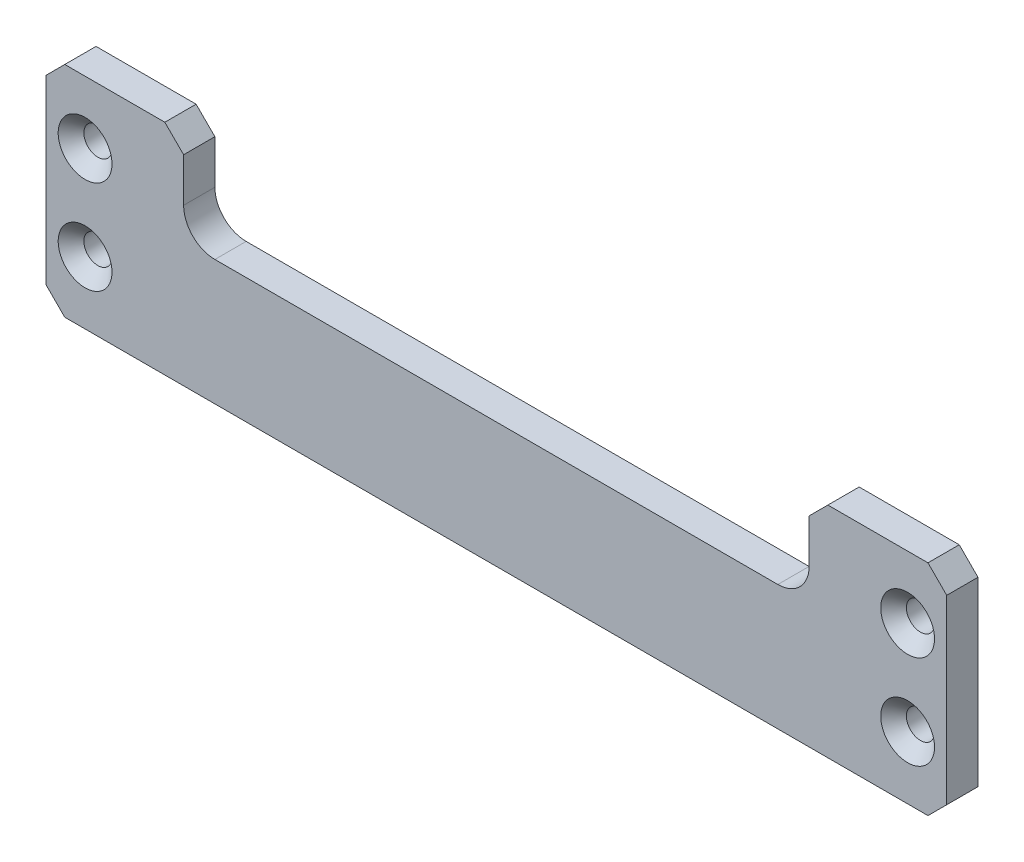
SolidWorks part; units mm, degrees
material "A6061"
ref_plane "前视基准面" through (0, 0, 0) normal (0, 0, 1) x (1, 0, 0)
ref_plane "上视基准面" through (0, 0, 0) normal (0, 1, 0) x (1, 0, 0)
ref_plane "右视基准面" through (0, 0, 0) normal (1, 0, 0) x (0, 0, -1)
sketch "草图1" plane through (0, 0, 0) normal (0, 0, 1) x (1, 0, 0)
  line L1 (-72, -17.5) -> (72, -17.5)
  line L2 (-72, -17.5) -> (-72, 17.5)
  line L3 (-72, 17.5) -> (72, 17.5)
  line L4 (72, -17.5) -> (72, 17.5)
  line L5 (-72, -17.5) -> (72, 17.5) construction
  line L6 (-72, 17.5) -> (72, -17.5) construction
  point P0 (0, 0)
  dimension "D1" = 35
  dimension "D2" = 144
extrude "凸台-拉伸1" add sketch "草图1" along normal blind 5
hole_wizard "打孔尺寸根据十字槽沉头木螺钉的类型1" positions "草图3" profile "草图2" countersink size "M4" standard "Gb" end condition through all
sketch "草图3" plane through (0, 0, 5) normal (0, 0, 1) x (1, 0, 0)
  line L0 (0, 0) -> (0, 17.5) construction
  line L1 (72, 17.5) -> (-72, 17.5) construction
  line L2 (0, 0) -> (72, 0) construction
  line L3 (72, -17.5) -> (72, 17.5) construction
  point P0 (-65.75, 7.5)
  point P2 (-65.75, -7.5)
  point P4 (65.75, 7.5)
  point P6 (65.75, -7.5)
  dimension "D1" = 131.5
  dimension "D2" = 15
sketch "草图2" plane through (-65.75, 7.5, 5) normal (1, 0, 0) x (0, -1, 0)
  line L0 (0, 0) -> (0, 5)
  line L1 (0, 5) -> (2.25, 5)
  line L2 (2.25, 5) -> (2.25, 2.05)
  line L3 (2.25, 2.05) -> (4.3, 0)
  line L5 (4.3, 0) -> (0, 0)
  line L6 (-2.25, 2.05) -> (-4.3, 0) construction
  line L11 (0, -6.35) -> (0, 107.95) construction
  dimension "通孔孔直径" = 4.5
  dimension "通孔孔深度" = 5
  dimension "近端锥形沉头孔直径" = 8.6
  dimension "近端锥形沉头孔角度" = 90
sketch "草图4" plane through (0, 0, 5) normal (0, 0, 1) x (1, 0, 0)
  line L0 (72, 17.5) -> (-72, 17.5) construction
  line L1 (-50, 17.5) -> (50, 17.5)
  line L2 (-50, 17.5) -> (-50, 2.5)
  line L3 (-50, 2.5) -> (50, 2.5)
  line L4 (50, 17.5) -> (50, 2.5)
  line L5 (0, 0) -> (0, 2.5) construction
  dimension "D1" = 15
  dimension "D2" = 100
extrude "切除-拉伸1" cut sketch "草图4" against normal through all
chamfer "倒角1" distance 3 angle 45 6 edges at (72, 17.5, 2.5) (72, -17.5, 2.5) (-72, -17.5, 2.5) (-72, 17.5, 2.5) (50, 17.5, 2.5) (-50, 17.5, 2.5)
fillet "圆角1" radius 5 2 edges at (50, 2.5, 2.5) (-50, 2.5, 2.5)
